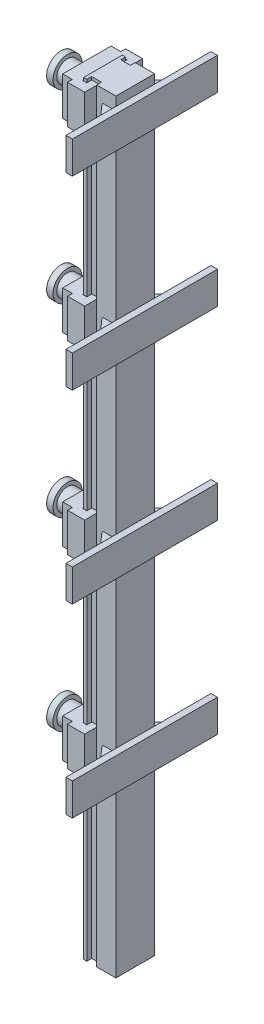
from build123d import *

# Parameters (mm, degrees)
BOSS_EXTRUDE1_DEPTH    = 2330
BOSS_EXTRUDE2_DEPTH    = 6
LPATTERN1_COUNT        = 2
LPATTERN1_PITCH        = 50
BOSS_EXTRUDE3_DEPTH    = 50
SKETCH4_R              = 17.5
BOSS_EXTRUDE4_DEPTH    = 2
BOSS_EXTRUDE5_DEPTH    = 12
LPATTERN2_COUNT        = 4
LPATTERN2_PITCH        = 575
LPATTERN2_COPY_1_DEPTH = 6
LPATTERN2_COPY_2_DEPTH = 6
LPATTERN2_COPY_3_DEPTH = 6
LPATTERN2_COPY_4_DEPTH = 50
LPATTERN2_COPY_5_DEPTH = 50
LPATTERN2_COPY_6_DEPTH = 50
BOSS_EXTRUDE6_DEPTH    = 60
SKETCH7_W              = 450
SKETCH7_H              = 100
BOSS_EXTRUDE7_DEPTH    = 20
BOSS_EXTRUDE8_DEPTH    = 40
LPATTERN5_COUNT        = 4
LPATTERN5_PITCH        = 575
SKETCH10_R             = 33.513199957
BOSS_EXTRUDE9_DEPTH    = 60
SKETCH11_R             = 45
BOSS_EXTRUDE10_DEPTH   = 20


with BuildPart() as part:
    # Sketch1 → Boss-Extrude1 (new body)
    with BuildSketch(Plane(origin=(0, 0, 0), x_dir=(1, 0, 0), z_dir=(0, 1, 0))):
        Polygon((10, 0), (10, -15), (40, -15), (40, 0), (100, 0), (100, -120), (40, -120), (40, -105), (10, -105), (10, -120), (0, -120), (0, 0), align=None)
    extrude(amount=BOSS_EXTRUDE1_DEPTH)

    # Sketch2 → Boss-Extrude2 (add)
    with BuildSketch(Plane(origin=(0, 2330, 0), x_dir=(1, 0, 0), z_dir=(0, 1, 0))):
        Polygon((60, -120), (100, -120), (100, 0), (60, 0), (60, 3), (95, 43), (95, 60), (110, 60), (110, -180), (95, -180), (95, -163), (60, -123), align=None)
    boss_extrude2 = extrude(amount=-BOSS_EXTRUDE2_DEPTH)

    # LPattern1: Boss-Extrude2 ×2
    with Locations(*[(0, -i * LPATTERN1_PITCH, 0) for i in range(1, LPATTERN1_COUNT)]):
        add(boss_extrude2)

    # Sketch3 → Boss-Extrude3 (add)
    with BuildSketch(Plane(origin=(0, 2280, 0), x_dir=(1, 0, 0), z_dir=(0, 1, 0))):
        Polygon((60, 3), (98, 3), (98, 60), (110, 60), (110, 0), (60, 0), align=None)
    boss_extrude3 = extrude(amount=BOSS_EXTRUDE3_DEPTH)

    # Mirror1: Boss-Extrude3 across plane
    add(boss_extrude3.mirror(Plane.XY.offset(60)))

    # Sketch4 → Boss-Extrude4 (add)
    with BuildSketch(Plane(origin=(0, 0, -3), x_dir=(-1, 0, 0), z_dir=(0, 0, -1))):
        with Locations(Location((-79, 2302, 0), (0, 0, 180))):
            Circle(SKETCH4_R)
    boss_extrude4 = extrude(amount=BOSS_EXTRUDE4_DEPTH)

    # Sketch5 → Boss-Extrude5 (add)
    with BuildSketch(Plane(origin=(0, 0, -5), x_dir=(-1, 0, 0), z_dir=(0, 0, -1))):
        Polygon((-65.522801719, 2294.058430392), (-65.383799833, 2309.70081128), (-78.860998114, 2317.642380888), (-92.477198281, 2309.941569608), (-92.616200167, 2294.29918872), (-79.139001886, 2286.357619112), align=None)
    boss_extrude5 = extrude(amount=BOSS_EXTRUDE5_DEPTH)

    # LPattern2: Boss-Extrude2, Boss-Extrude3, Boss-Extrude4, Boss-Extrude5 ×4
    with Locations(*[(0, -i * LPATTERN2_PITCH, 0) for i in range(1, LPATTERN2_COUNT)]):
        add(boss_extrude2)
        add(boss_extrude3)
        add(boss_extrude4)
        add(boss_extrude5)

    # LPattern2 copy 1 sketch → LPattern2 copy 1 (add)
    with BuildSketch(Plane(origin=(0, 1705, 0), x_dir=(1, 0, 0), z_dir=(0, 1, 0))):
        Polygon((60, -120), (100, -120), (100, 0), (60, 0), (60, 3), (95, 43), (95, 60), (110, 60), (110, -180), (95, -180), (95, -163), (60, -123), align=None)
    extrude(amount=-LPATTERN2_COPY_1_DEPTH)

    # LPattern2 copy 2 sketch → LPattern2 copy 2 (add)
    with BuildSketch(Plane(origin=(0, 1130, 0), x_dir=(1, 0, 0), z_dir=(0, 1, 0))):
        Polygon((60, -120), (100, -120), (100, 0), (60, 0), (60, 3), (95, 43), (95, 60), (110, 60), (110, -180), (95, -180), (95, -163), (60, -123), align=None)
    extrude(amount=-LPATTERN2_COPY_2_DEPTH)

    # LPattern2 copy 3 sketch → LPattern2 copy 3 (add)
    with BuildSketch(Plane(origin=(0, 555, 0), x_dir=(1, 0, 0), z_dir=(0, 1, 0))):
        Polygon((60, -120), (100, -120), (100, 0), (60, 0), (60, 3), (95, 43), (95, 60), (110, 60), (110, -180), (95, -180), (95, -163), (60, -123), align=None)
    extrude(amount=-LPATTERN2_COPY_3_DEPTH)

    # LPattern2 copy 4 sketch → LPattern2 copy 4 (add)
    with BuildSketch(Plane(origin=(0, 1705, 120), x_dir=(1, 0, 0), z_dir=(0, 1, 0))):
        Polygon((60, -3), (98, -3), (98, -60), (110, -60), (110, 0), (60, 0), align=None)
    extrude(amount=LPATTERN2_COPY_4_DEPTH)

    # LPattern2 copy 5 sketch → LPattern2 copy 5 (add)
    with BuildSketch(Plane(origin=(0, 1130, 120), x_dir=(1, 0, 0), z_dir=(0, 1, 0))):
        Polygon((60, -3), (98, -3), (98, -60), (110, -60), (110, 0), (60, 0), align=None)
    extrude(amount=LPATTERN2_COPY_5_DEPTH)

    # LPattern2 copy 6 sketch → LPattern2 copy 6 (add)
    with BuildSketch(Plane(origin=(0, 555, 120), x_dir=(1, 0, 0), z_dir=(0, 1, 0))):
        Polygon((60, -3), (98, -3), (98, -60), (110, -60), (110, 0), (60, 0), align=None)
    extrude(amount=LPATTERN2_COPY_6_DEPTH)

    # Sketch7 → Boss-Extrude7 (add)
    with BuildSketch(Plane(origin=(110, 0, 0), x_dir=(0, 0, -1), z_dir=(1, 0, 0))):
        with Locations((-60, 2302)):
            Rectangle(SKETCH7_W, SKETCH7_H)
    boss_extrude7 = extrude(amount=BOSS_EXTRUDE7_DEPTH)

    # Sketch8 → Boss-Extrude8 (add)
    with BuildSketch(Plane(origin=(0, 2330, 0), x_dir=(1, 0, 0), z_dir=(0, 1, 0))):
        Polygon((0, 0), (10, 0), (10, -15), (40, -15), (40, 0), (100, 0), (100, -120), (40, -120), (40, -105), (10, -105), (10, -120), (0, -120), align=None)
    extrude(amount=BOSS_EXTRUDE8_DEPTH)


with BuildPart() as body_2:
    # Sketch6 → Boss-Extrude6 (new, symmetric)
    with BuildSketch(Plane(origin=(0, 2302, 0), x_dir=(1, 0, 0), z_dir=(0, 1, 0))):
        Polygon((33.129061176, 30), (33.129061176, -13.291657706), (11.568777139, -13.291657706), (11.568777139, 2.446888421), (-1.368841287, 2.446888421), (-1.368841287, -121.695701217), (11.568777139, -121.695701217), (11.568777139, -106.165445456), (33.129061176, -106.165445456), (33.129061176, -150), (-20, -150), (-20, -135), (-50, -135), (-50, 15), (-20, 15), (-20, 30), align=None)
    boss_extrude6 = extrude(amount=BOSS_EXTRUDE6_DEPTH, both=True)

    # Sketch10 → Boss-Extrude9 (add)
    with BuildSketch(Plane.ZY.offset(50)):
        with Locations((60, 2302)):
            Circle(SKETCH10_R)
        with Locations((60, 1727)):
            Circle(SKETCH10_R)
        with Locations((60, 1152)):
            Circle(SKETCH10_R)
        with Locations((60, 577)):
            Circle(SKETCH10_R)
    extrude(amount=BOSS_EXTRUDE9_DEPTH)


with BuildPart() as part_1:
    add(part.part)

    # LPattern5: Boss-Extrude6, Boss-Extrude7 ×4
    with Locations(*[(0, -i * LPATTERN5_PITCH, 0) for i in range(1, LPATTERN5_COUNT)]):
        add(boss_extrude6)
        add(boss_extrude7)


with BuildPart() as boss_extrude9_piece_1:
    # of the separate pieces the step leaves, piece 1, a body of its own (boss_extrude9_pieces)
    add(body_2.part.solids().sort_by_distance((33.129061176, 2242, -30))[0])



with BuildPart() as boss_extrude9_piece_2:
    # of the separate pieces the step leaves, piece 2, a body of its own (boss_extrude9_pieces)
    add(body_2.part.solids().sort_by_distance((-50, 1152, 93.513199957))[0])


with BuildPart() as boss_extrude9_piece_3:
    # of the separate pieces the step leaves, piece 3, a body of its own (boss_extrude9_pieces)
    add(body_2.part.solids().sort_by_distance((-50, 577, 93.513199957))[0])


with BuildPart() as boss_extrude9_piece_4:
    # of the separate pieces the step leaves, piece 4, a body of its own (boss_extrude9_pieces)
    add(body_2.part.solids().sort_by_distance((-50, 1727, 93.513199957))[0])


with BuildPart() as boss_extrude9_piece_1_1:
    add(boss_extrude9_piece_1.part)

    add(boss_extrude9_piece_2.part)  # Boss-Extrude10 merges Boss-Extrude9 piece 2

    add(boss_extrude9_piece_3.part)  # Boss-Extrude10 merges Boss-Extrude9 piece 3

    add(boss_extrude9_piece_4.part)  # Boss-Extrude10 merges Boss-Extrude9 piece 4
    # Sketch11 → Boss-Extrude10 (add)
    with BuildSketch(Plane.ZY.offset(110)):
        with Locations((60, 2302)):
            Circle(SKETCH11_R)
        with Locations((60, 1727)):
            Circle(SKETCH11_R)
        with Locations((60, 1152)):
            Circle(SKETCH11_R)
        with Locations((60, 577)):
            Circle(SKETCH11_R)
    extrude(amount=BOSS_EXTRUDE10_DEPTH)


solid = Compound([part_1.part, boss_extrude9_piece_1_1.part])
